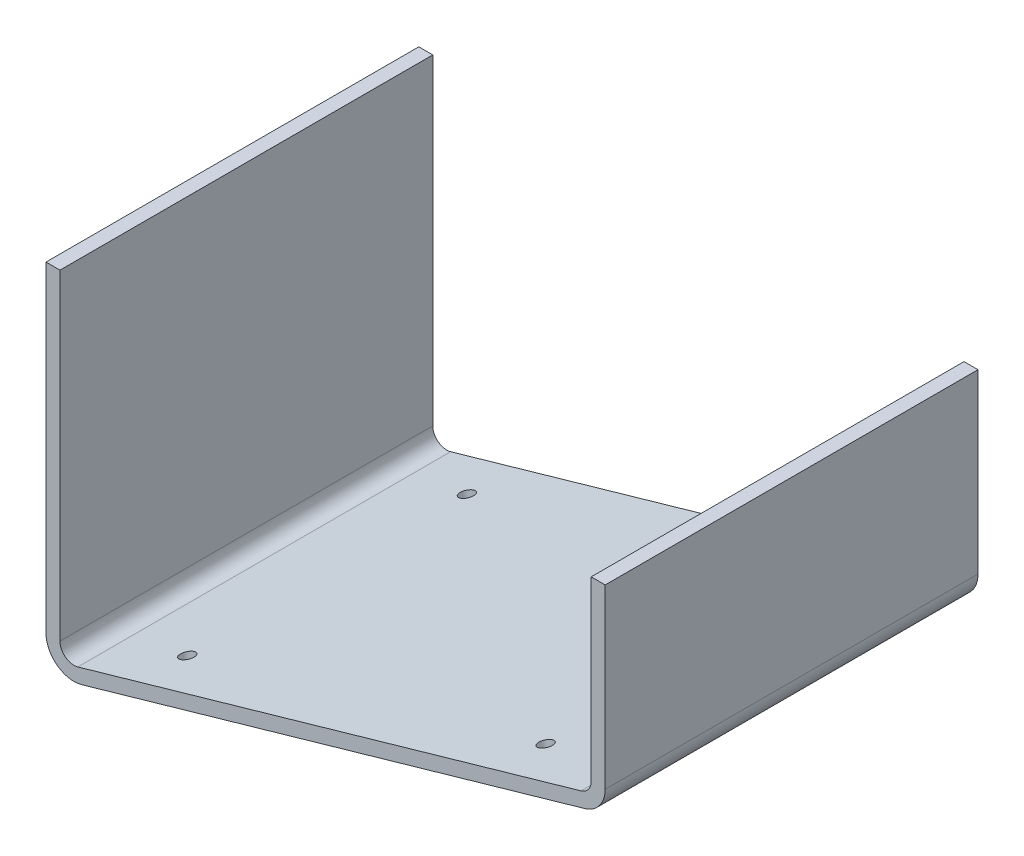
SolidWorks part; units mm, degrees
material "1023 carbon steel plate (SS)"
ref_plane "Front Plane" through (0, 0, 0) normal (0, 0, 1) x (1, 0, 0)
ref_plane "Top Plane" through (0, 0, 0) normal (0, 1, 0) x (1, 0, 0)
ref_plane "Right Plane" through (0, 0, 0) normal (1, 0, 0) x (0, 0, -1)
sketch "Sketch1" plane through (0, 0, 0) normal (0, 0, 1) x (1, 0, 0)
  line L0 (0, 0) -> (0, -137.8944)
  line L2 (240, -75.9574) -> (240, 0)
  line L4 (15.3076, -149.4295) -> (231.3076, -87.4925)
  line L5 (6, 0) -> (6, -137.8944)
  line L6 (13.6538, -143.6619) -> (229.6538, -81.7249)
  line L7 (234, -75.9574) -> (234, 0)
  line L8 (6, 0) -> (0, 0)
  line L9 (234, 0) -> (240, 0)
  line L10 (0, -153.8189) -> (240, -85) construction
  line L11 (240, -85) -> (240, 0) construction
  line L12 (0, 0) -> (0, -153.8189) construction
  line L13 (6, -145.8566) -> (234, -80.4787) construction
  line L14 (234, -80.4787) -> (234, 0) construction
  line L15 (6, 0) -> (6, -145.8566) construction
  arc A0 (231.3076, -87.4925) -> (240, -75.9574) centre (228, -75.9574) ccw
  arc A1 (0, -137.8944) -> (15.3076, -149.4295) centre (12, -137.8944) ccw
  arc A2 (229.6538, -81.7249) -> (234, -75.9574) centre (228, -75.9574) ccw
  arc A3 (6, -137.8944) -> (13.6538, -143.6619) centre (12, -137.8944) ccw
  point P13 (240, -85)
  dimension "D5" = 12
  dimension "D1" = 6
  dimension "D2" = 16
  dimension "D4" = 85
  dimension "D3" = 6
extrude "Boss-Extrude1" add sketch "Sketch1" along normal blind 160 contours L9 L2 A0 L4 A1 L0 L8 L5 A3 L6 A2 L7
sketch "Sketch2" plane through (40.7558, -142.1324, 0) normal (0.2756, -0.9613, 0) x (0.9613, 0.2756, 0)
  line L0 (-26.4737, 160) -> (198.231, 160) construction
  line L1 (-42.3982, 160) -> (-42.3982, 0) construction
  circle A0 centre (1.6018, 140) radius 3
  circle A1 centre (1.6018, 20) radius 3
  circle A2 centre (161.6018, 140) radius 3
  circle A3 centre (161.6018, 20) radius 3
  dimension "D3" = 6
  dimension "D4" = 20
  dimension "D5" = 44
  dimension "D1" = 160
  dimension "D2" = 120
extrude "Cut-Extrude1" cut sketch "Sketch2" against normal blind 8
